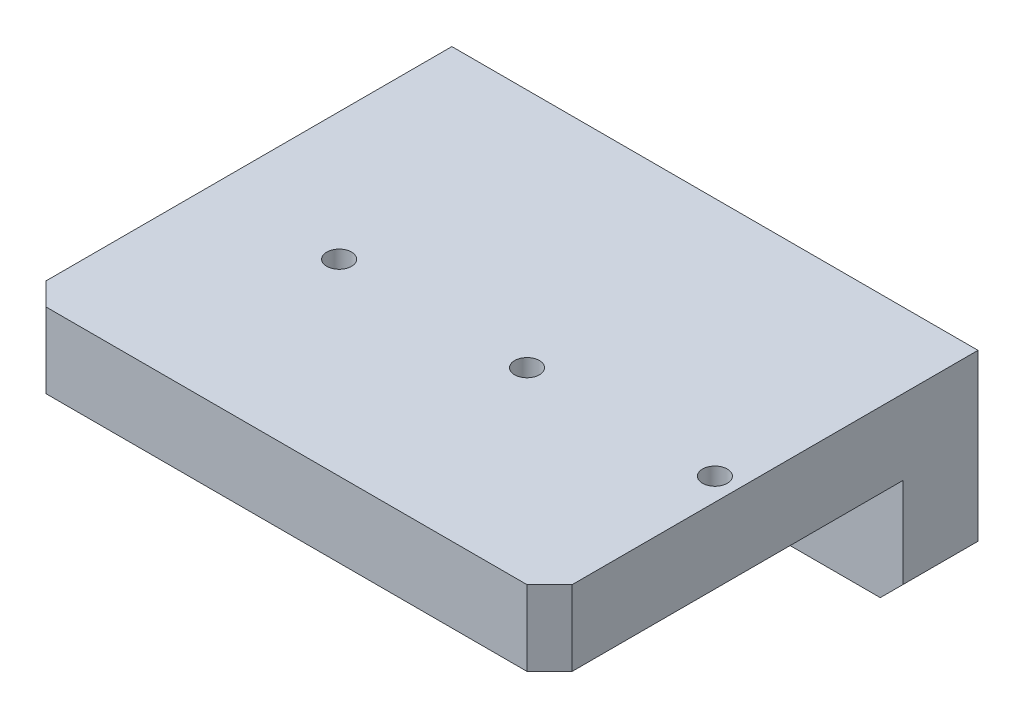
from build123d import *

# Parameters (mm, degrees)
SKETCH_1_W                  = 70
SKETCH_1_H                  = 57
EXTRUDE_1_DEPTH             = 10
SKETCH_2_W                  = 70
SKETCH_2_H                  = 10
EXTRUDE_2_DEPTH             = 15
CHAMFER_1_SIZE              = 3
HOLE_WIZARD_M4_1_D          = 3.3
HOLE_WIZARD_M4_1_DEPTH      = 10.1
HOLE_WIZARD_M4_1_TIP        = 0.991420021
HOLE_WIZARD_5_5_5_5_1_D     = 5.5
HOLE_WIZARD_5_5_5_5_1_DEPTH = 10.1
HOLE_WIZARD_5_5_5_5_1_TIP   = 1.652366702


with BuildPart() as part:
    # 草图1 → 凸台-拉伸1 (new body)
    with BuildSketch(Plane(origin=(0, 0, 0), x_dir=(1, 0, 0), z_dir=(0, 1, 0))):
        Rectangle(SKETCH_1_W, SKETCH_1_H)
    extrude(amount=EXTRUDE_1_DEPTH)

    # 草图2 → 凸台-拉伸2 (add)
    with BuildSketch(Plane.XZ):
        with Locations((0, -23.5)):
            Rectangle(SKETCH_2_W, SKETCH_2_H)
    extrude(amount=EXTRUDE_2_DEPTH)

    # 倒角1
    chamfer_1_edges = [part.edges().sort_by_distance(p)[0] for p in [
        (35, -15, -23.5),
        (-35, -15, -23.5),
        (35, 5, 28.5),
        (-35, 5, 28.5),
    ]]
    chamfer(chamfer_1_edges, length=CHAMFER_1_SIZE)

    # M4 螺纹孔1
    with Locations(Plane(origin=(0, 10, 0), x_dir=(1, 0, 0), z_dir=(0, 1, 0))):
        with Locations((32, -3.5), (-18, -3.5), (7, -3.5)):
            Hole(HOLE_WIZARD_M4_1_D / 2, depth=HOLE_WIZARD_M4_1_DEPTH)
            with Locations((0, 0, -(HOLE_WIZARD_M4_1_DEPTH + HOLE_WIZARD_M4_1_TIP / 2))):  # 118° drill point
                Cone(0, HOLE_WIZARD_M4_1_D / 2, HOLE_WIZARD_M4_1_TIP, mode=Mode.SUBTRACT)

    # Ø5.5 (5.5) 直径孔1
    with Locations(Plane.XY.offset(-18.5)):
        with Locations((-15, -7.5), (-30, -7.5)):
            Hole(HOLE_WIZARD_5_5_5_5_1_D / 2, depth=HOLE_WIZARD_5_5_5_5_1_DEPTH)
            with Locations((0, 0, -(HOLE_WIZARD_5_5_5_5_1_DEPTH + HOLE_WIZARD_5_5_5_5_1_TIP / 2))):  # 118° drill point
                Cone(0, HOLE_WIZARD_5_5_5_5_1_D / 2, HOLE_WIZARD_5_5_5_5_1_TIP, mode=Mode.SUBTRACT)


solid = part.part
